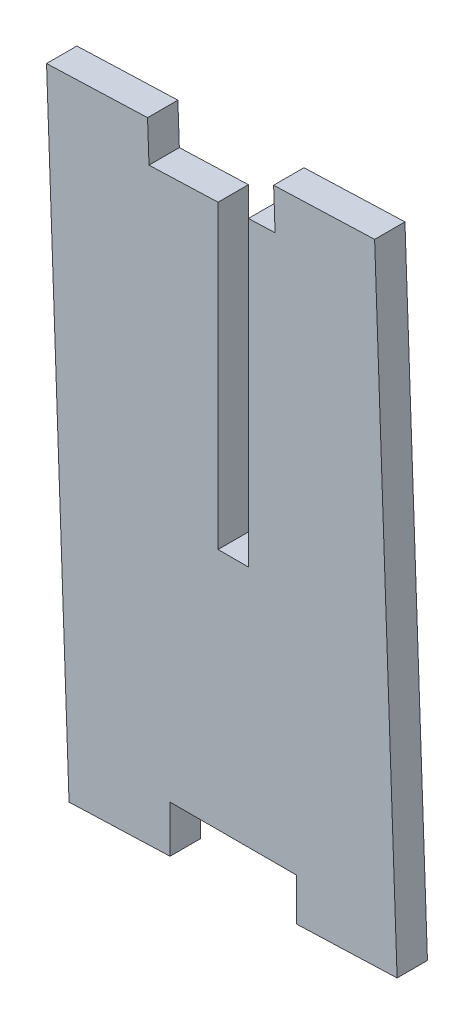
from build123d import *

# Parameters (mm, degrees)
BOSS_EXTRUDE1_DEPTH = 6
SKETCH2_W           = 6
SKETCH2_H           = 59.975118876
CUT_EXTRUDE1_DEPTH  = 6


with BuildPart() as part:
    # Sketch1 → Boss-Extrude1 (new body)
    with BuildSketch(Plane.XY):
        Polygon((107.036449202, -34.108774603), (102.587015051, 90.196105325), (122.563832413, 90.911166016), (122.850005344, 82.916286089), (147.788760974, 83.808957004), (147.502588043, 91.803836932), (167.479405405, 92.518897623), (171.928839556, -31.785982304), (152.013983639, -32.498825115), (152.013983639, -24.108777743), (127.013266564, -24.108777743), (127.013266564, -33.393713911), align=None)
    extrude(amount=BOSS_EXTRUDE1_DEPTH)

    # Sketch2 → Cut-Extrude1 (cut)
    with BuildSketch(Plane.XY.offset(6)):
        with Locations((139.513625101, 53.898004923)):
            Rectangle(SKETCH2_W, SKETCH2_H)
    extrude(amount=-CUT_EXTRUDE1_DEPTH, mode=Mode.SUBTRACT)


solid = part.part
